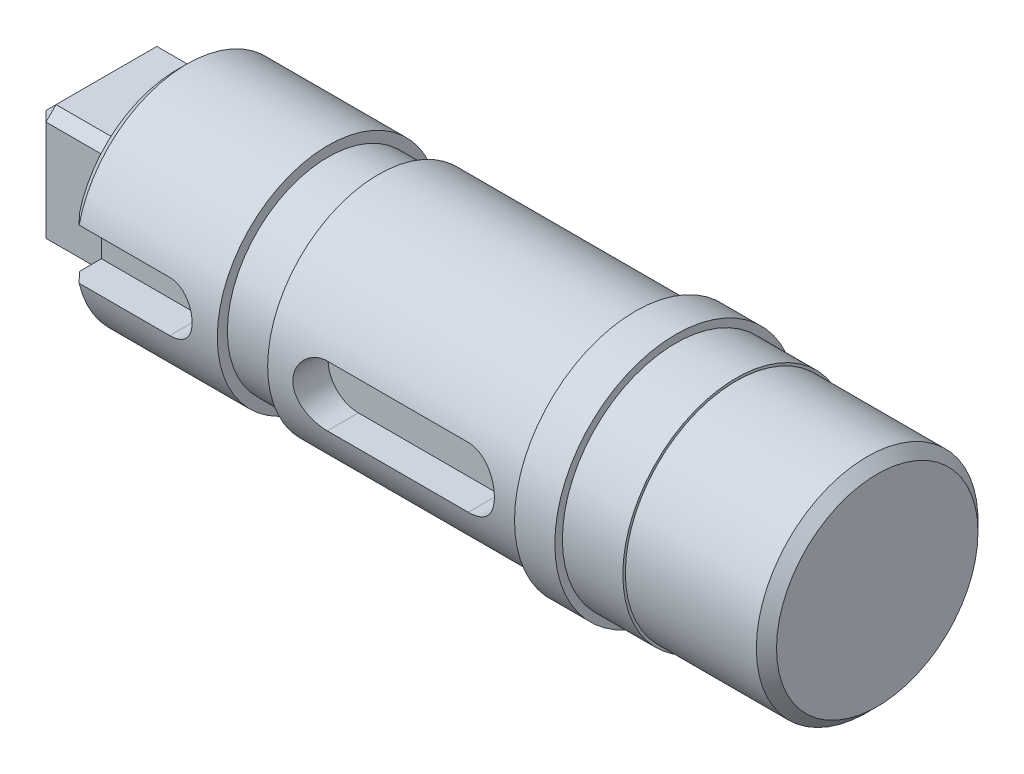
from build123d import *

# Parameters (mm, degrees)
SKETCH2_W           = 12
SKETCH2_H           = 12
BOSS_EXTRUDE1_DEPTH = 8
CHAMFER1_SIZE       = 1
CUT_EXTRUDE1_DEPTH  = 3.5
CUT_EXTRUDE2_DEPTH  = 3.5


with BuildPart() as part:
    # Sketch1 → Revolve1 (revolve)
    with BuildSketch(Plane.XY, mode=Mode.PRIVATE) as revolve1_sk:
        Polygon((-41.365727984, 0), (28.134272016, 0), (28.134272016, 11), (14.134272016, 11), (14.134272016, 11.25), (8.134272016, 11.25), (8.134272016, 12), (4.134272016, 12), (4.134272016, 11), (-21.365727984, 11), (-21.365727984, 10), (-26.365727984, 10), (-26.365727984, 11), (-41.365727984, 11), align=None)
    revolve(revolve1_sk.sketch.rotate(Axis((-41.365727984, 0, 0), (1, 0, 0)), 90), axis=Axis((-41.365727984, 0, 0), (1, 0, 0)))

    # Sketch2 → Boss-Extrude1 (add)
    with BuildSketch(Plane.ZY.offset(41.365727984)):
        Rectangle(SKETCH2_W, SKETCH2_H)
    extrude(amount=BOSS_EXTRUDE1_DEPTH)

    # Chamfer1
    chamfer1_edges = [part.edges().sort_by_distance(p)[0] for p in [
        (-41.365727984, 0, -11),
        (28.134272016, 0, -11),
        (-45.365727984, -6, 6),
        (-45.365727984, 6, 6),
        (-45.365727984, 6, -6),
        (-45.365727984, -6, -6),
        (-49.365727984, 0, 6),
        (-49.365727984, 6, 0),
        (-49.365727984, 0, -6),
        (-49.365727984, -6, 0),
    ]]
    chamfer(chamfer1_edges, length=CHAMFER1_SIZE)

    # Sketch3 → Cut-Extrude1 (cut)
    with BuildSketch(Plane.XY.offset(11)):
        with BuildLine():
            Line((-15.865727984, 3), (-1.865727984, 3))
            ThreePointArc((-1.865727984, 3), (1.134272016, 0), (-1.865727984, -3))
            Line((-1.865727984, -3), (-15.865727984, -3))
            ThreePointArc((-15.865727984, -3), (-18.865727984, 0), (-15.865727984, 3))
        make_face()
    extrude(amount=-CUT_EXTRUDE1_DEPTH, mode=Mode.SUBTRACT)

    # Sketch4 → Cut-Extrude2 (cut)
    with BuildSketch(Plane.XY.offset(11)):
        with BuildLine():
            Line((-41.365727984, -2.5), (-31.365727984, -2.5))
            ThreePointArc((-31.365727984, -2.5), (-28.865727984, 0), (-31.365727984, 2.5))
            Line((-31.365727984, 2.5), (-41.365727984, 2.5))
            Line((-41.365727984, 2.5), (-41.365727984, -2.5))
        make_face()
    extrude(amount=-CUT_EXTRUDE2_DEPTH, mode=Mode.SUBTRACT)


solid = part.part
